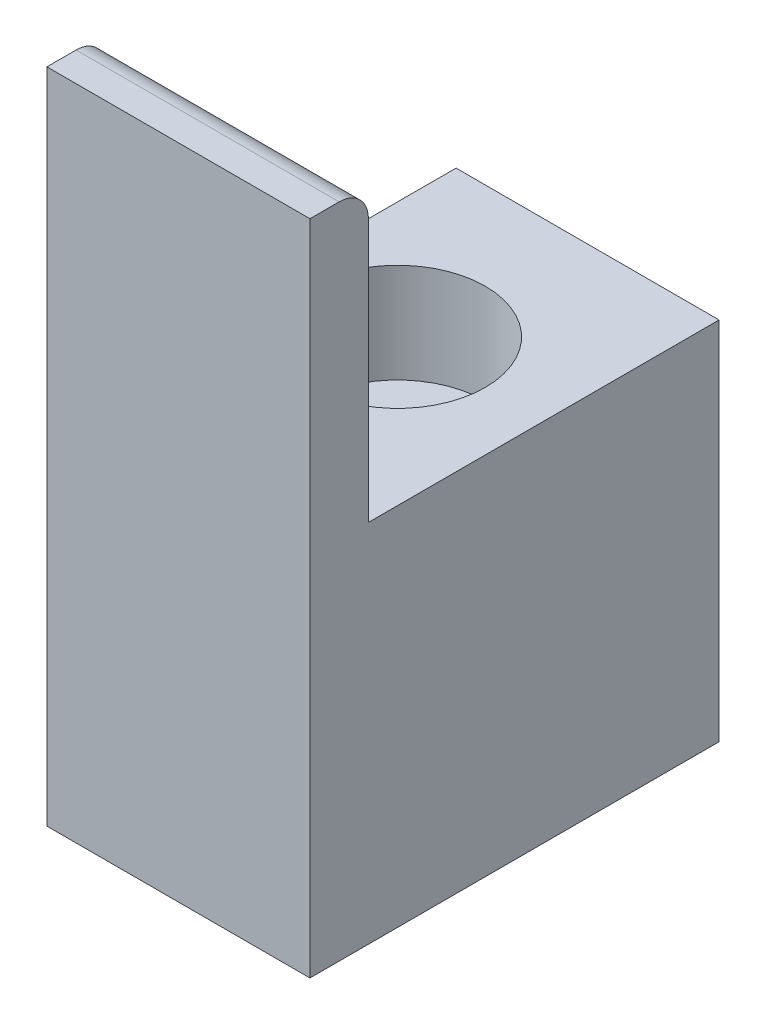
SolidWorks part; units mm, degrees
ref_plane "Front Plane" through (0, 0, 0) normal (0, 0, 1) x (1, 0, 0)
ref_plane "Top Plane" through (0, 0, 0) normal (0, 1, 0) x (1, 0, 0)
ref_plane "Right Plane" through (0, 0, 0) normal (1, 0, 0) x (0, 0, -1)
sketch "Sketch1" plane through (0, 0, 0) normal (0, 1, 0) x (1, 0, 0)
  line L1 (-4.5, 7) -> (4.5, 7)
  line L2 (-4.5, 7) -> (-4.5, -7)
  line L3 (-4.5, -7) -> (4.5, -7)
  line L4 (4.5, 7) -> (4.5, -7)
  line L5 (-4.5, 7) -> (4.5, -7) construction
  line L6 (-4.5, -7) -> (4.5, 7) construction
  point P0 (0, 0)
  dimension "D1" = 9
  dimension "D2" = 14
extrude "Boss-Extrude1" add sketch "Sketch1" along normal blind 12.5
sketch "Sketch2" plane through (0, 0, 0) normal (0, -1, 0) x (1, 0, 0)
  line L2 (1, 1) -> (-2, 1)
  line L3 (-2, -3) -> (1, -3)
  line L4 (1, 1) -> (-2, 1)
  line L5 (-2, -3) -> (1, -3)
  arc A2 (-2, 1) -> (-2, -3) centre (-0.5, -1) ccw
  arc A3 (1, -3) -> (1, 1) centre (-0.5, -1) ccw
  arc A4 (-2, 1) -> (-2, -3) centre (-0.5, -1) ccw
  arc A5 (1, -3) -> (1, 1) centre (-0.5, -1) ccw
  dimension "D1" = 0
extrude "Cut-Extrude1" cut sketch "Sketch2" against normal blind 3
sketch "Sketch3" plane through (0, 0, 7) normal (0, 0, 1) x (1, 0, 0)
  line L0 (4.5, 12.5) -> (4.5, 0) construction
  line L1 (-4.5, 12.5) -> (4.5, 12.5)
  line L2 (-4.5, 12.5) -> (-4.5, 22.5)
  line L3 (-4.5, 22.5) -> (4.5, 22.5)
  line L4 (4.5, 12.5) -> (4.5, 22.5)
  dimension "D1" = 10
extrude "Boss-Extrude2" add sketch "Sketch3" against normal blind 2
fillet "Fillet1" radius 1 1 edges at (0, 22.5, 5)
sketch "Sketch4" plane through (0, 12.5, 0) normal (0, 1, 0) x (1, 0, 0)
  point P0 (-0.5, 1)
hole_wizard "Hole size (per hex socket screw type) 1" positions "3DSketch1" profile "Sketch5" counterbore size "M3" standard "GB" end condition through all
sketch3d "3DSketch1"
  point P0 (-0.5, 12.5, -1)
sketch "Sketch5" plane through (-0.5, 12.5, -1) normal (1, 0, 0) x (0, 0, 1)
  line L0 (0, 0) -> (0, 12.5)
  line L1 (0, 12.5) -> (1.7, 12.5)
  line L3 (1.7, 12.5) -> (1.7, 3.4)
  line L4 (1.7, 3.4) -> (3, 3.4)
  line L5 (3, 3.4) -> (3, 0)
  line L7 (3, 0) -> (0, 0)
  line L11 (0, -6.35) -> (0, 107.95) construction
  dimension "通孔孔直径" = 3.4
  dimension "通孔孔深度" = 12.5
  dimension "柱形沉头孔直径" = 6
  dimension "柱形沉头孔深度" = 3.4
